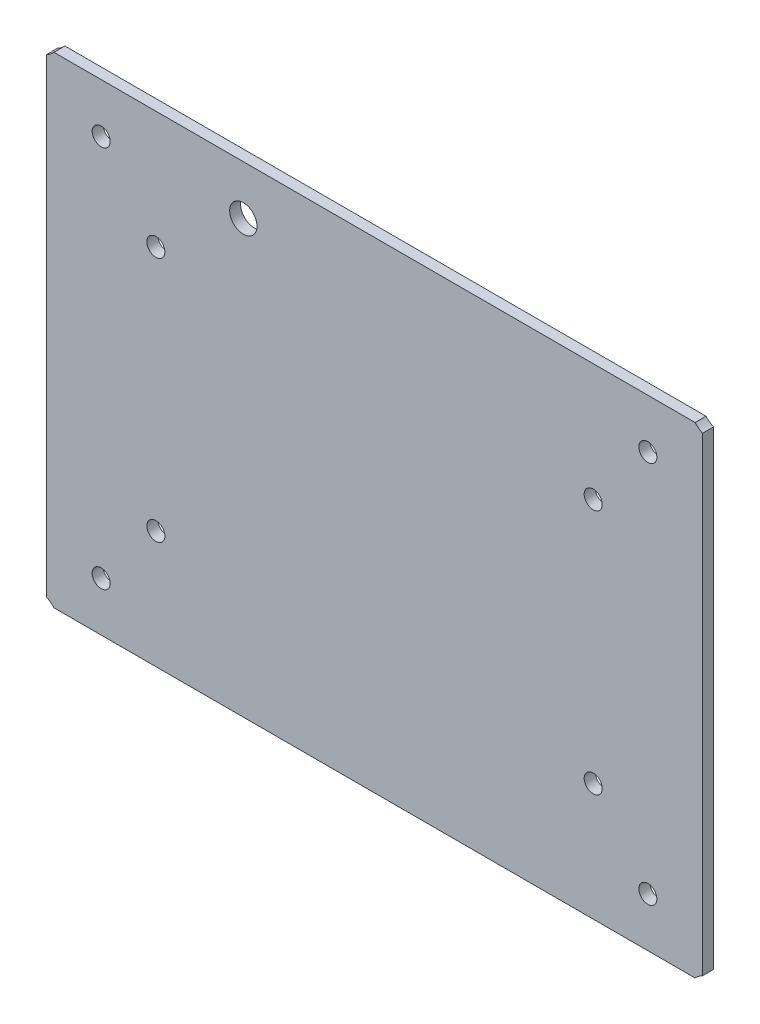
from build123d import *

# Parameters (mm, degrees)
SKETCH_1_W          = 120
SKETCH_1_H          = 88
SKETCH_1_R          = 1.65
SKETCH_1_R_2        = 2.5
EXTRUDE_1_DEPTH     = 1
SKETCH_2_R          = 4.5
CUT_EXTRUDE_1_DEPTH = 2.5


with BuildPart() as part:
    # 草图1 → 凸台-拉伸1 (new, symmetric)
    with BuildSketch(Plane.XY):
        Rectangle(SKETCH_1_W, SKETCH_1_H)
        with Locations((-40, -22.5)):
            Circle(SKETCH_1_R, mode=Mode.SUBTRACT)
        with Locations((-40, 22.5)):
            Circle(SKETCH_1_R, mode=Mode.SUBTRACT)
        with Locations((40, -22.5)):
            Circle(SKETCH_1_R, mode=Mode.SUBTRACT)
        with Locations((40, 22.5)):
            Circle(SKETCH_1_R, mode=Mode.SUBTRACT)
        with Locations((-50, -35)):
            Circle(SKETCH_1_R, mode=Mode.SUBTRACT)
        with Locations((-50, 35)):
            Circle(SKETCH_1_R, mode=Mode.SUBTRACT)
        with Locations((50, -35)):
            Circle(SKETCH_1_R, mode=Mode.SUBTRACT)
        with Locations((50, 35)):
            Circle(SKETCH_1_R, mode=Mode.SUBTRACT)
        with Locations((-24, 35)):
            Circle(SKETCH_1_R_2, mode=Mode.SUBTRACT)
    extrude(amount=EXTRUDE_1_DEPTH, both=True)

    # 草图2 → 切除-拉伸1 (cut, symmetric)
    with BuildSketch(Plane.XY):
        with Locations((-62, -47)):
            Circle(SKETCH_2_R)
        with Locations((-62, 47)):
            Circle(SKETCH_2_R)
        with Locations((62, -47)):
            Circle(SKETCH_2_R)
        with Locations((62, 47)):
            Circle(SKETCH_2_R)
    extrude(amount=CUT_EXTRUDE_1_DEPTH, both=True, mode=Mode.SUBTRACT)


solid = part.part
